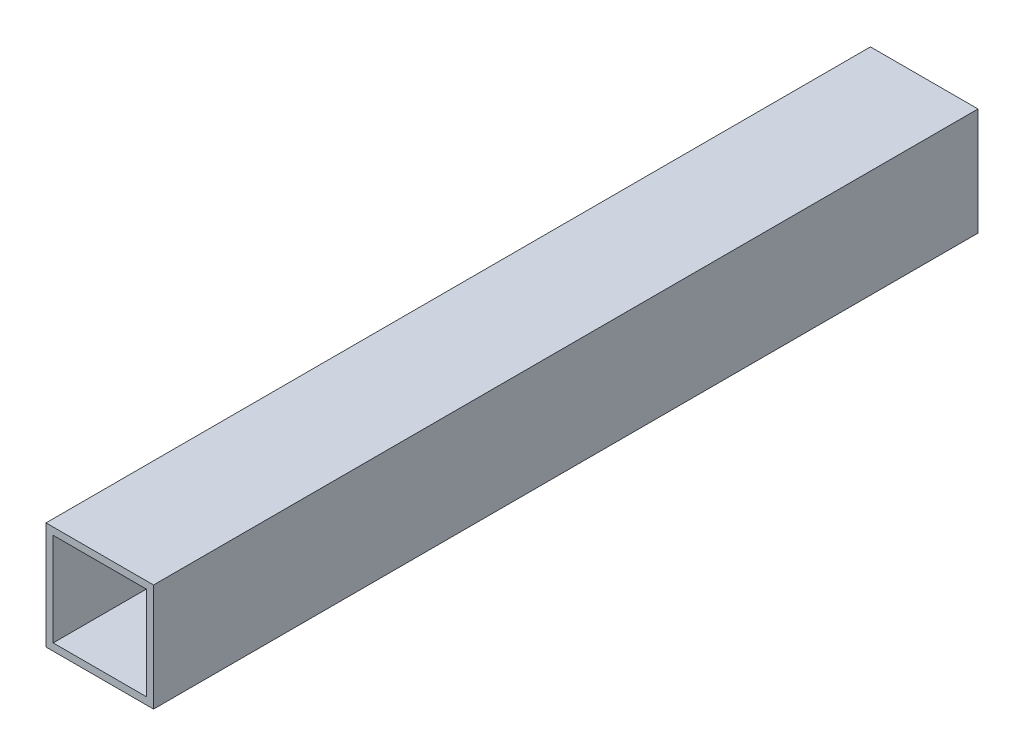
SolidWorks part; units mm, degrees
ref_plane "前视基准面" through (0, 0, 0) normal (0, 0, 1) x (1, 0, 0)
ref_plane "上视基准面" through (0, 0, 0) normal (0, 1, 0) x (1, 0, 0)
ref_plane "右视基准面" through (0, 0, 0) normal (1, 0, 0) x (0, 0, -1)
sketch "草图1" plane through (0, 0, 0) normal (0, 0, 1) x (1, 0, 0)
  line L0 (13, -13) -> (13, 13)
  line L1 (15, -15) -> (-15, -15)
  line L2 (15, -15) -> (15, 15)
  line L3 (15, 15) -> (-15, 15)
  line L4 (-15, -15) -> (-15, 15)
  line L5 (15, -15) -> (-15, 15) construction
  line L6 (15, 15) -> (-15, -15) construction
  line L7 (13, 13) -> (-13, 13)
  line L8 (-13, -13) -> (-13, 13)
  line L9 (13, -13) -> (-13, -13)
  point P0 (0, 0)
  dimension "D1" = 30
  dimension "D2" = 2
extrude "凸台-拉伸1" add sketch "草图1" along normal mid plane 230
sketch "草图2" plane through (0, 0, 115) normal (0, 0, 1) x (1, 0, 0)
  circle A1 centre (0, 0) radius 4.2683
